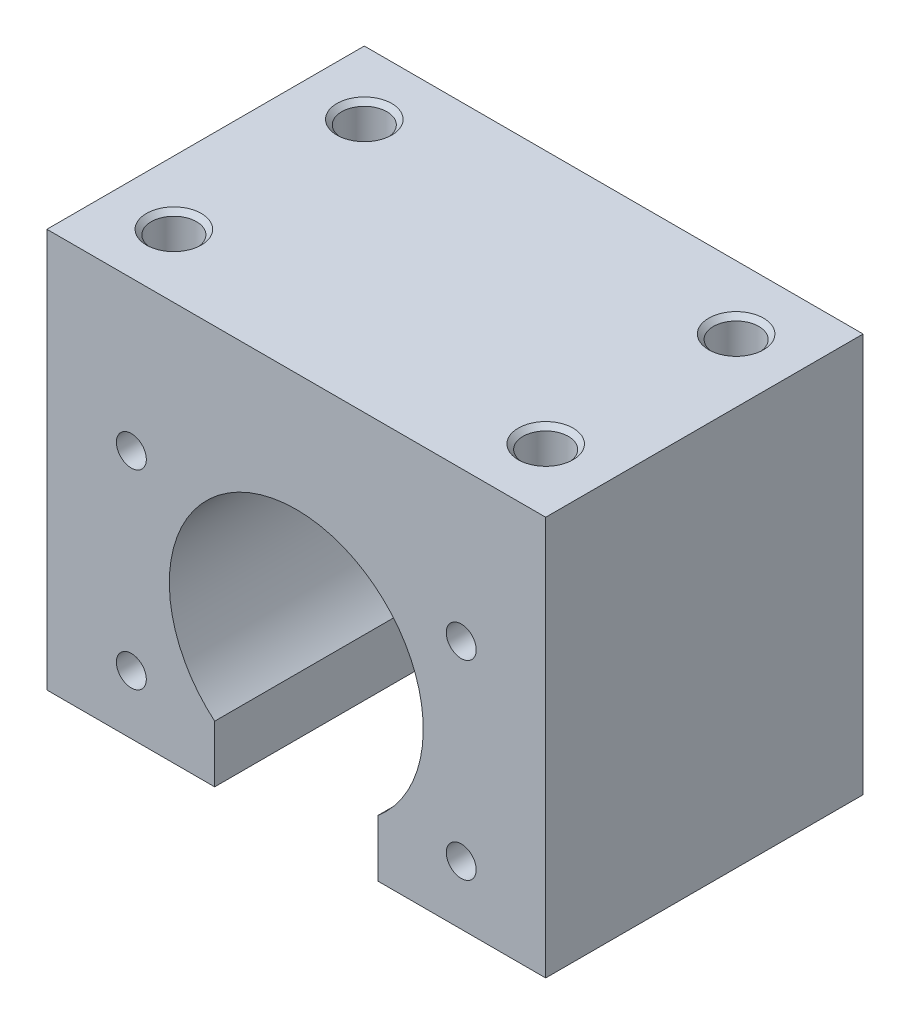
SolidWorks part; units mm, degrees
ref_plane "前视基准面" through (0, 0, 0) normal (0, 0, 1) x (1, 0, 0)
ref_plane "上视基准面" through (0, 0, 0) normal (0, 1, 0) x (1, 0, 0)
ref_plane "右视基准面" through (0, 0, 0) normal (1, 0, 0) x (0, 0, -1)
sketch "草图1" plane through (0, 0, 0) normal (0, 0, 1) x (1, 0, 0)
  line L0 (-27.5, 27) -> (27.5, 27)
  line L1 (27.5, 27) -> (27.5, -17)
  line L2 (27.5, -17) -> (9, -17)
  line L3 (9, -17) -> (9, -10.7238)
  line L4 (-27.5, 27) -> (-27.5, -17)
  line L5 (-27.5, -17) -> (-9, -17)
  line L6 (-9, -17) -> (-9, -10.7238)
  arc A0 (9, -10.7238) -> (-9, -10.7238) centre (0, 0) ccw
extrude "凸台-拉伸1" add sketch "草图1" along normal mid plane 35
hole_wizard "M4 螺纹孔1" positions "草图3" profile "草图2" tap size "M4" standard "GB"
sketch "草图3" plane through (0, 0, 17.5) normal (0, 0, 1) x (1, 0, 0)
  circle A0 centre (18.1865, 10.5) radius 2.25 construction
  circle A1 centre (18.1865, -10.5) radius 2.25 construction
  circle A2 centre (-18.1865, -10.5) radius 2.25 construction
  circle A3 centre (-18.1865, 10.5) radius 2.25 construction
  point P1 (18.1865, 10.5)
  point P5 (18.1865, -10.5)
  point P9 (-18.1865, -10.5)
  point P13 (-18.1865, 10.5)
cosmetic thread "孔螺蚊线1" parameters "D1"=6, "D2"=4
cosmetic thread "孔螺蚊线2" parameters "D1"=6, "D2"=4
cosmetic thread "孔螺蚊线3" parameters "D1"=6, "D2"=4
cosmetic thread "孔螺蚊线4" parameters "D1"=6, "D2"=4
sketch "草图2" plane through (18.1865, 10.5, 17.5) normal (1, 0, 0) x (0, -1, 0)
  line L0 (0, 0) -> (0, 10.4914)
  line L1 (0, 10.4914) -> (1.65, 9.5)
  line L2 (1.65, 9.5) -> (1.65, 0)
  line L5 (1.65, 0) -> (0, 0)
  line L10 (0, 10.4914) -> (-1.65, 9.5) construction
  line L11 (0, -6.35) -> (0, 107.95) construction
  dimension "螺纹孔钻头直径" = 3.3
  dimension "螺纹孔钻头深度" = 9.5
  dimension "导头角度" = 118
sketch "草图4" plane through (0, 27, 0) normal (0, 1, 0) x (1, 0, 0)
  line L0 (27.5, -17.5) -> (27.5, 17.5) construction
  line L1 (-20.5, -10.5) -> (20.5, -10.5)
  line L2 (-20.5, -10.5) -> (-20.5, 10.5)
  line L3 (-20.5, 10.5) -> (20.5, 10.5)
  line L4 (20.5, -10.5) -> (20.5, 10.5)
  line L5 (-20.5, -10.5) -> (20.5, 10.5) construction
  line L6 (-20.5, 10.5) -> (20.5, -10.5) construction
  line L7 (27.5, -17.5) -> (-27.5, -17.5) construction
  point P0 (0, 0)
  dimension "D1" = 7
  dimension "D2" = 7
hole_wizard "M6 螺纹孔1" positions "3D草图1" profile "草图5" tap size "M6" standard "GB"
sketch3d "3D草图1"
  point P0 (-20.5, 27, 10.5)
  point P3 (-20.5, 27, -10.5)
  point P6 (20.5, 27, -10.5)
  point P9 (20.5, 27, 10.5)
sketch "草图5" plane through (-20.5, 27, 10.5) normal (1, 0, 0) x (0, 0, 1)
  line L0 (0, 0) -> (0, 13.5022)
  line L1 (0, 13.5022) -> (2.5, 12)
  line L2 (2.5, 12) -> (2.5, 0.525)
  line L3 (2.5, 0.525) -> (3.025, 0)
  line L5 (3.025, 0) -> (0, 0)
  line L6 (-2.5, 0.525) -> (-3.025, 0) construction
  line L10 (0, 13.5022) -> (-2.5, 12) construction
  line L11 (0, -6.35) -> (0, 107.95) construction
  dimension "螺纹孔钻头直径" = 5
  dimension "螺纹孔钻头深度" = 12
  dimension "近端锥形沉头孔直径" = 6.05
  dimension "近端锥形沉头孔角度" = 90
  dimension "导头角度" = 118
cosmetic thread "孔螺蚊线5" parameters "D1"=8, "D2"=6
cosmetic thread "孔螺蚊线6" parameters "D1"=8, "D2"=6
cosmetic thread "孔螺蚊线7" parameters "D1"=8, "D2"=6
cosmetic thread "孔螺蚊线8" parameters "D1"=8, "D2"=6
equation "\"D3@草图1\"=\"D2@草图1\""
